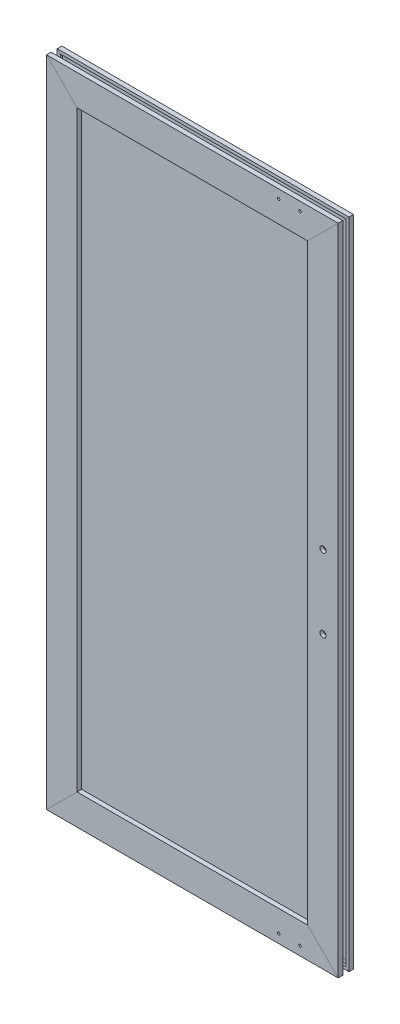
SolidWorks part; units mm, degrees
material "铝型材"
ref_plane "前视基准面" through (0, 0, 0) normal (0, 0, 1) x (1, 0, 0)
ref_plane "上视基准面" through (0, 0, 0) normal (0, 1, 0) x (1, 0, 0)
ref_plane "右视基准面" through (0, 0, 0) normal (1, 0, 0) x (0, 0, -1)
sketch "草图13" plane through (0, 0, 0) normal (0, 0, 1) x (1, 0, 0)
  line L1 (-171, -408) -> (171, -408)
  line L2 (-171, -408) -> (-171, 408)
  line L3 (-171, 408) -> (171, 408)
  line L4 (171, -408) -> (171, 408)
  line L5 (-171, -408) -> (171, 408) construction
  line L6 (-171, 408) -> (171, -408) construction
  point P0 (0, 0)
  dimension "D1" = 342
  dimension "D2" = 816
other "铝型材 2040A(1)"
ref_plane "基准面3" through (-171, 408, 0) normal (1, 0, 0) x (0, 1, 0)
sketch "草图19" plane through (-171, 408, 0) normal (1, 0, 0) x (0, 1, 0)
  line L0 (9, 4) -> (6, 4)
  line L1 (9, 4) -> (9, 7)
  line L2 (6, -4) -> (6, 4)
  line L3 (16, 7) -> (9, 7)
  line L4 (9, -4) -> (6, -4)
  line L5 (16, 4) -> (16, 7)
  line L6 (9, -7) -> (9, -4)
  line L7 (20, 4) -> (16, 4)
  line L8 (16, -7) -> (9, -7)
  line L9 (20, 10) -> (20, 4)
  line L10 (16, -7) -> (16, -4)
  line L11 (-20, 10) -> (20, 10)
  line L12 (20, -4) -> (16, -4)
  line L13 (-20, 4) -> (-20, 10)
  line L14 (20, -4) -> (20, -10)
  line L15 (-20, 4) -> (-16, 4)
  line L16 (20, -10) -> (-20, -10)
  line L17 (-16, 4) -> (-16, 7)
  line L18 (-20, -10) -> (-20, -4)
  line L19 (-16, 7) -> (-9, 7)
  line L20 (-20, -4) -> (-16, -4)
  line L21 (-9, 4) -> (-9, 7)
  line L22 (-16, -7) -> (-16, -4)
  line L23 (-9, 4) -> (-6, 4)
  line L24 (-16, -7) -> (-9, -7)
  line L25 (-6, -4) -> (-6, 4)
  line L26 (-9, -7) -> (-9, -4)
  line L27 (-9, -4) -> (-6, -4)
  circle A0 centre (0, 0) radius 3.25
  point P0 (0, 0)
sketch "草图14" plane through (0, 0, 0) normal (0, 0, 1) x (1, 0, 0)
  line L0 (177, 414) -> (180, 417) construction
  line L1 (-164.5, -401.5) -> (164.5, -401.5)
  line L2 (-164.5, -401.5) -> (-164.5, 401.5)
  line L3 (-164.5, 401.5) -> (164.5, 401.5)
  line L4 (164.5, -401.5) -> (164.5, 401.5)
  line L5 (-164.5, -401.5) -> (164.5, 401.5) construction
  line L6 (-164.5, 401.5) -> (164.5, -401.5) construction
  line L8 (151, 388) -> (-151, 388) construction
  point P0 (0, 0)
  dimension "D1" = 13.5
extrude "凸台-拉伸1" add sketch "草图14" along normal mid plane 4 separate body
hole_wizard "M4 螺纹孔2" positions "草图24" profile "草图25" tap size "M4" standard "GB"
sketch "草图24" plane through (0, 0, 10) normal (0, 0, -1) x (-1, 0, 0)
  line L0 (-141, 416.5) -> (-113, 416.5) construction
  line L7 (0, 0) -> (81.0682, 0) construction
  line L10 (-191, 428) -> (191, 428) construction
  line L11 (-191, -428) -> (-191, 428) construction
  point P0 (-141, 416.5)
  point P2 (-113, 416.5)
  point P29 (-113, -416.5)
  point P30 (-141, -416.5)
  dimension "D1" = 28
  dimension "D2" = 11.5
  dimension "D3" = 50
cosmetic thread "孔螺蚊线3"
cosmetic thread "孔螺蚊线4"
cosmetic thread "孔螺蚊线9"
cosmetic thread "孔螺蚊线10"
sketch "草图25" plane through (141, 416.5, 10) normal (1, 0, 0) x (0, -1, 0)
  line L0 (0, 0) -> (0, 11.0914)
  line L1 (0, 11.0914) -> (1.65, 10.1)
  line L2 (1.65, 10.1) -> (1.65, 0)
  line L5 (1.65, 0) -> (0, 0)
  line L10 (0, 11.0914) -> (-1.65, 10.1) construction
  line L11 (0, -6.35) -> (0, 107.95) construction
  dimension "螺纹孔钻头直径" = 3.3
  dimension "螺纹孔钻头深度" = 10.1
  dimension "导头角度" = 118
hole_wizard "打孔尺寸(%根据)开槽圆柱头螺钉的类型1" positions "草图26" profile "草图27" counterbore size "M4" standard "GB" end condition through all
sketch "草图26" plane through (0, 0, 10) normal (0, 0, 1) x (1, 0, 0)
  line L0 (0, 0) -> (50000, 0) construction
  line L1 (171, 424) -> (171, -49576) construction
  line L2 (191, 428) -> (151, 388) construction
  point P0 (171, 48)
  point P2 (171, -48)
  point P14 (171, 408)
  dimension "D1" = 96
sketch "草图27" plane through (171, 48, 10) normal (1, 0, 0) x (0, -1, 0)
  line L0 (0, 0) -> (0, 20)
  line L1 (0, 20) -> (2.25, 20)
  line L3 (2.25, 20) -> (2.25, 4.6)
  line L4 (2.25, 4.6) -> (4, 4.6)
  line L5 (4, 4.6) -> (4, 0)
  line L7 (4, 0) -> (0, 0)
  line L11 (0, -6.35) -> (0, 107.95) construction
  dimension "通孔孔直径" = 4.5
  dimension "通孔孔深度" = 20
  dimension "柱形沉头孔直径" = 8
  dimension "柱形沉头孔深度" = 4.6
hole_wizard "M6 螺纹孔1" positions "草图28" profile "草图29" tap size "M6" standard "GB"
sketch "草图28" plane through (0, 0, -10) normal (0, 0, -1) x (-1, 0, 0)
  line L0 (0, 0) -> (50000, 0) construction
  line L1 (171, 424) -> (171, -49576) construction
  line L2 (151, 388) -> (191, 428) construction
  line L3 (-191, 428) -> (191, 428) construction
  line L4 (171, -469.5) -> (171, 49530.5) construction
  point P0 (171, 368)
  point P2 (171, 331)
  point P12 (171, 408)
  point P19 (171, -368)
  point P20 (171, -331)
  dimension "D1" = 60
  dimension "D2" = 37
sketch "草图29" plane through (-171, 368, -10) normal (1, 0, 0) x (0, 1, 0)
  line L0 (0, 0) -> (0, 18.5022)
  line L1 (0, 18.5022) -> (2.5, 17)
  line L2 (2.5, 17) -> (2.5, 0)
  line L5 (2.5, 0) -> (0, 0)
  line L10 (0, 18.5022) -> (-2.5, 17) construction
  line L11 (0, -6.35) -> (0, 107.95) construction
  dimension "螺纹孔钻头直径" = 5
  dimension "螺纹孔钻头深度" = 17
  dimension "导头角度" = 118
cosmetic thread "孔螺蚊线5"
cosmetic thread "孔螺蚊线6"
cosmetic thread "孔螺蚊线7"
cosmetic thread "孔螺蚊线8"
